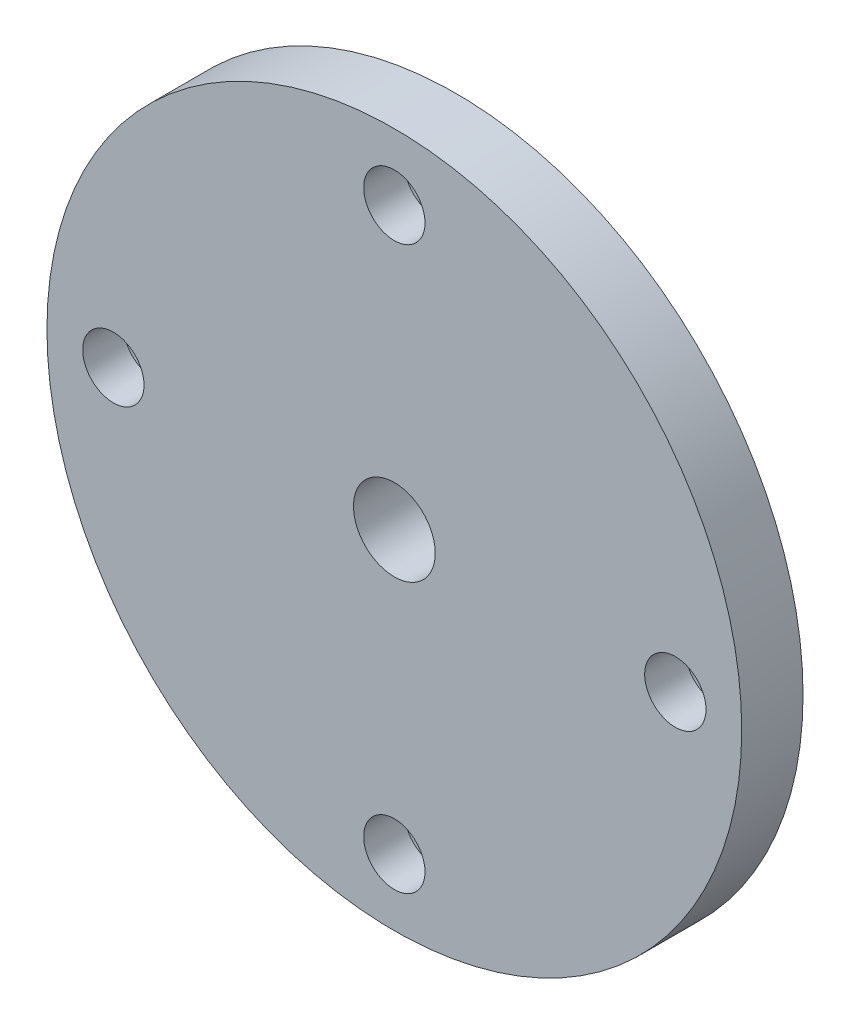
from build123d import *

# Parameters (mm, degrees)
SKETCH1_R           = 34
BOSS_EXTRUDE1_DEPTH = 6
SKETCH2_R           = 3
CUT_EXTRUDE1_DEPTH  = 4
SKETCH3_R           = 4
CUT_EXTRUDE2_DEPTH  = 49.456165758


with BuildPart() as part:
    # Sketch1 → Boss-Extrude1 (new body)
    with BuildSketch(Plane.XY):
        Circle(SKETCH1_R)
    extrude(amount=BOSS_EXTRUDE1_DEPTH)

    # Sketch2 → Cut-Extrude1 (cut)
    with BuildSketch(Plane.XY.offset(6)):
        with Locations((0, 27.5)):
            Circle(SKETCH2_R)
        with Locations((27.5, 0)):
            Circle(SKETCH2_R)
        with Locations((0, -27.5)):
            Circle(SKETCH2_R)
        with Locations((-27.5, 0)):
            Circle(SKETCH2_R)
    extrude(amount=-CUT_EXTRUDE1_DEPTH, mode=Mode.SUBTRACT)

    # Sketch3 → Cut-Extrude2 (cut, through all)
    with BuildSketch(Plane.XY.offset(6)):
        Circle(SKETCH3_R)
    extrude(amount=-CUT_EXTRUDE2_DEPTH, mode=Mode.SUBTRACT)


solid = part.part
